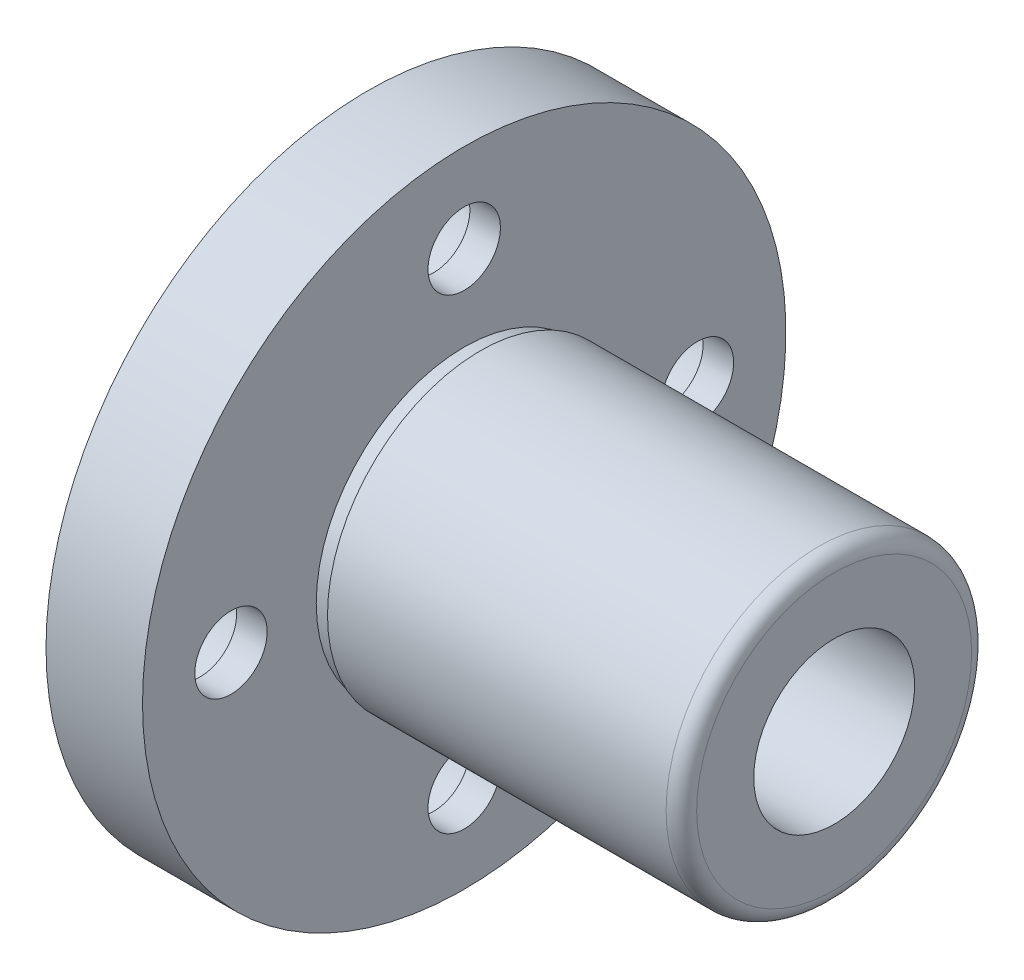
SolidWorks part; units mm, degrees
ref_plane "前视基准面" through (0, 0, 0) normal (0, 0, 1) x (1, 0, 0)
ref_plane "上视基准面" through (0, 0, 0) normal (0, 1, 0) x (1, 0, 0)
ref_plane "右视基准面" through (0, 0, 0) normal (1, 0, 0) x (0, 0, -1)
sketch "草图1" plane through (0, 0, 0) normal (0, 0, 1) x (1, 0, 0)
  line L0 (0, 20) -> (0, 5)
  line L1 (0, 5) -> (29, 5)
  line L2 (29, 5) -> (29, 8.55)
  line L3 (28.05, 9.5) -> (7, 9.5)
  line L4 (7, 9.5) -> (7, 9.2)
  line L5 (7, 9.2) -> (6, 9.2)
  line L6 (6, 9.2) -> (6, 20)
  line L7 (6, 20) -> (0, 20)
  line L8 (29, 0) -> (0, 0) construction
  arc A0 (29, 8.55) -> (28.05, 9.5) centre (28.05, 8.55) ccw
revolve "旋转1" add sketch "草图1" angle 360 about L8
sketch "草图2" plane through (0, 0, 0) normal (0, 0, 1) x (1, 0, 0)
  line L0 (0, 14.5) -> (0, 18.25)
  line L1 (0, 18.25) -> (4.1, 18.25)
  line L2 (4.1, 18.25) -> (4.1, 16.75)
  line L3 (4.1, 16.75) -> (6, 16.75)
  line L4 (6, 16.75) -> (6, 14.5)
  line L5 (6, 14.5) -> (0, 14.5)
  line L6 (6, 14.5) -> (0, 14.5) construction
revolve "切除-旋转1" cut sketch "草图2" angle 360 about L6
sketch "草图3" plane through (0, 0, 0) normal (1, 0, 0) x (0, 0, -1)
  line L0 (0, 14.5) -> (-707.1068, -692.6068)
  line L1 (0, 14.5) -> (707.1068, -692.6068)
pattern_linear "阵列(线性)1" count 2 spacing 20.5061 along (0, -0.7071, 0.7071) count 2 spacing 20.5061 along (0, -0.7071, -0.7071) of "切除-旋转1"
